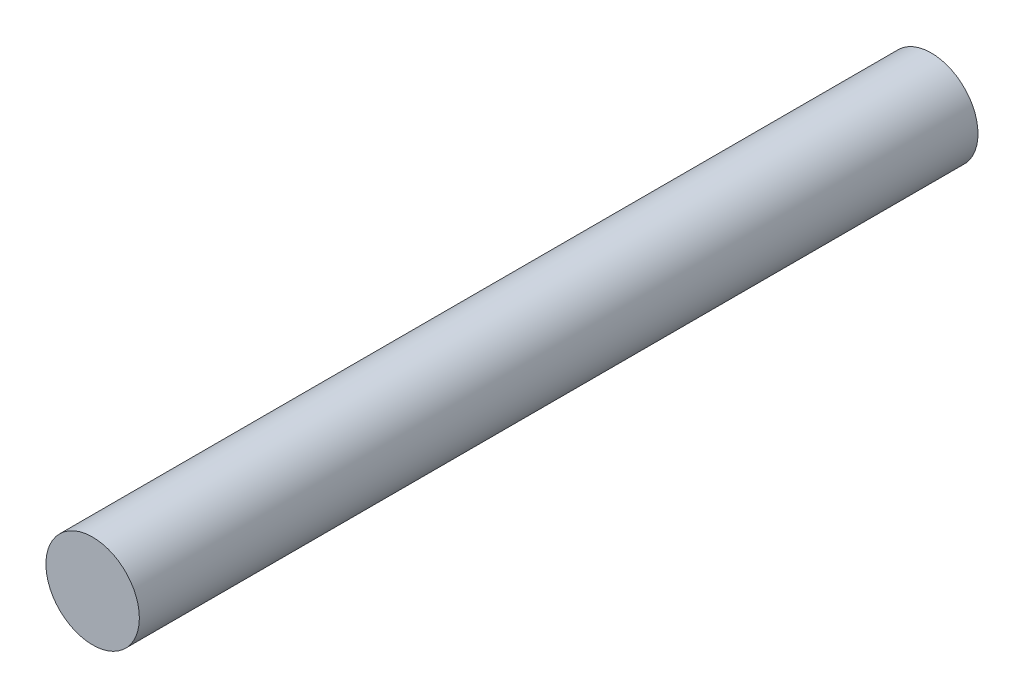
from build123d import *

# Parameters (mm, degrees)
SKETCH1_R           = 3.9
BOSS_EXTRUDE1_DEPTH = 70


with BuildPart() as part:
    # Sketch1 → Boss-Extrude1 (new body)
    with BuildSketch(Plane.XY):
        with Locations((8, -61.753173354)):
            Circle(SKETCH1_R)
    extrude(amount=BOSS_EXTRUDE1_DEPTH)


solid = part.part
